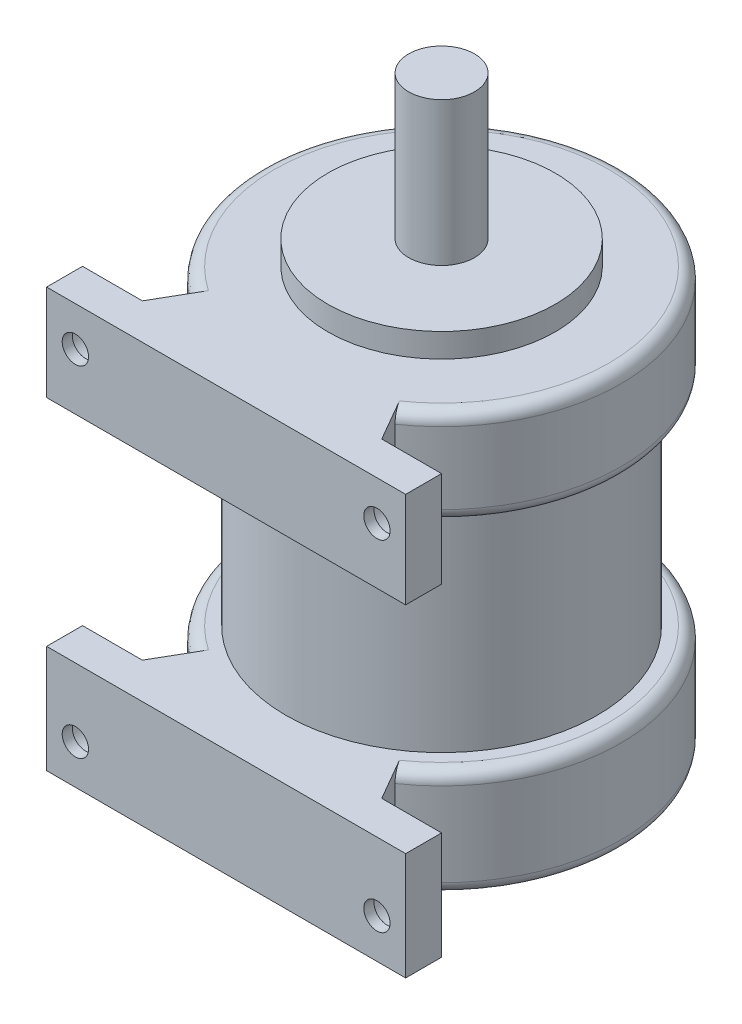
from build123d import *

# Parameters (mm, degrees)
SKETCH_1_R               = 150
EXTRUDE_1_DEPTH          = 350
EXTRUDE_2_DEPTH          = 350
SKETCH_3_R               = 95
EXTRUDE_3_DEPTH          = 20
CUT_EXTRUDE_START        = -80
SKETCH_4_OUTSIDE_W       = 417.896
SKETCH_4_OUTSIDE_H       = 447.896
SKETCH_4_OUTSIDE_R       = 130
CUT_EXTRUDE_1_DEPTH      = 180
FILLET_1_R               = 10
SKETCH_5_R               = 27.5
EXTRUDE_4_DEPTH          = 120
HOLE_WIZARD_1_AT_2_COUNT = 2
HOLE_WIZARD_1_AT_2_PITCH = 284
HOLE_WIZARD_1_AT_3_COUNT = 2
HOLE_WIZARD_1_AT_3_PITCH = 379.684079203
HOLE_WIZARD_1_AT_4_COUNT = 2
HOLE_WIZARD_1_AT_4_PITCH = 252


with BuildPart() as part:
    # 草图1 → 凸台-拉伸1 (new body)
    with BuildSketch(Plane(origin=(0, 0, 0), x_dir=(1, 0, 0), z_dir=(0, 1, 0))):
        with Locations(Location((0, 0, 0), (0, 0, 270))):
            Circle(SKETCH_1_R)
    extrude(amount=EXTRUDE_1_DEPTH)

    # 草图2 → 凸台-拉伸2 (add)
    with BuildSketch(Plane.XZ):
        with BuildLine():
            Line((-84.823393206, 123.713345946), (-100, 150))
            Line((-100, 150), (-150, 150))
            Line((-150, 150), (-150, 180))
            Line((-150, 180), (150, 180))
            Line((150, 180), (150, 150))
            Line((150, 150), (100, 150))
            Line((100, 150), (84.823393206, 123.713345946))
            ThreePointArc((84.823393206, 123.713345946), (0, 150), (-84.823393206, 123.713345946))
        make_face()
    extrude(amount=-EXTRUDE_2_DEPTH)

    # 草图3 → 凸台-拉伸3 (add)
    with BuildSketch(Plane(origin=(0, 350, 0), x_dir=(1, 0, 0), z_dir=(0, 1, 0))):
        with Locations(Location((0, 0, 0), (0, 0, 270))):
            Circle(SKETCH_3_R)
    extrude(amount=EXTRUDE_3_DEPTH)

    # 草图4 outside → 切除-拉伸1 (cut)
    with BuildSketch(Plane(origin=(0, 350, 0), x_dir=(1, 0, 0), z_dir=(0, 1, 0)).offset(CUT_EXTRUDE_START)):
        with Locations((0, -15)):
            Rectangle(SKETCH_4_OUTSIDE_W, SKETCH_4_OUTSIDE_H)
        with Locations(Location((0, 0, 0), (0, 0, 270))):
            Circle(SKETCH_4_OUTSIDE_R, mode=Mode.SUBTRACT)
    extrude(amount=-CUT_EXTRUDE_1_DEPTH, mode=Mode.SUBTRACT)

    # 圆角1
    fillet_1_edges = [part.edges().sort_by_distance(p)[0] for p in [
        (0, 0, -150),
        (0, 350, -150),
        (0, 270, -150),
        (0, 90, -150),
    ]]
    fillet(fillet_1_edges, radius=FILLET_1_R)

    # 草图7 → 打孔尺寸(%根据)内六角圆柱头螺钉的类型1 (revolve, cut)
    with BuildSketch(Plane(origin=(126, 317, 150), x_dir=(0, 1, 0), z_dir=(1, 0, 0))):
        Polygon((0, 0), (0, 30), (11, 30), (11, 21.5), (16.5, 21.5), (16.5, 0), align=None)
    hole_wizard_1 = revolve(axis=Axis((126, 317, 143.65), (0, 0, 1)), mode=Mode.SUBTRACT)

    # 打孔尺寸(%根据)内六角圆柱头螺钉的类型1 at 2: 打孔尺寸(%根据)内六角圆柱头螺钉的类型1 ×2
    with Locations(*[(0, -i * HOLE_WIZARD_1_AT_2_PITCH, 0) for i in range(1, HOLE_WIZARD_1_AT_2_COUNT)]):
        add(hole_wizard_1, mode=Mode.SUBTRACT)

    # 打孔尺寸(%根据)内六角圆柱头螺钉的类型1 at 3: 打孔尺寸(%根据)内六角圆柱头螺钉的类型1 ×2
    with Locations(*[Vector(-0.6637096834009412, -0.747990278118521, 0) * (i * HOLE_WIZARD_1_AT_3_PITCH) for i in range(1, HOLE_WIZARD_1_AT_3_COUNT)]):
        add(hole_wizard_1, mode=Mode.SUBTRACT)

    # 打孔尺寸(%根据)内六角圆柱头螺钉的类型1 at 4: 打孔尺寸(%根据)内六角圆柱头螺钉的类型1 ×2
    with Locations(*[(-i * HOLE_WIZARD_1_AT_4_PITCH, 0, 0) for i in range(1, HOLE_WIZARD_1_AT_4_COUNT)]):
        add(hole_wizard_1, mode=Mode.SUBTRACT)


with BuildPart() as body_2:
    # 草图5 → 凸台-拉伸4 (new body)
    with BuildSketch(Plane(origin=(0, 370, 0), x_dir=(1, 0, 0), z_dir=(0, 1, 0))):
        with Locations(Location((0, 0, 0), (0, 0, 90))):
            Circle(SKETCH_5_R)
    extrude(amount=EXTRUDE_4_DEPTH)


solid = Compound([part.part, body_2.part])
